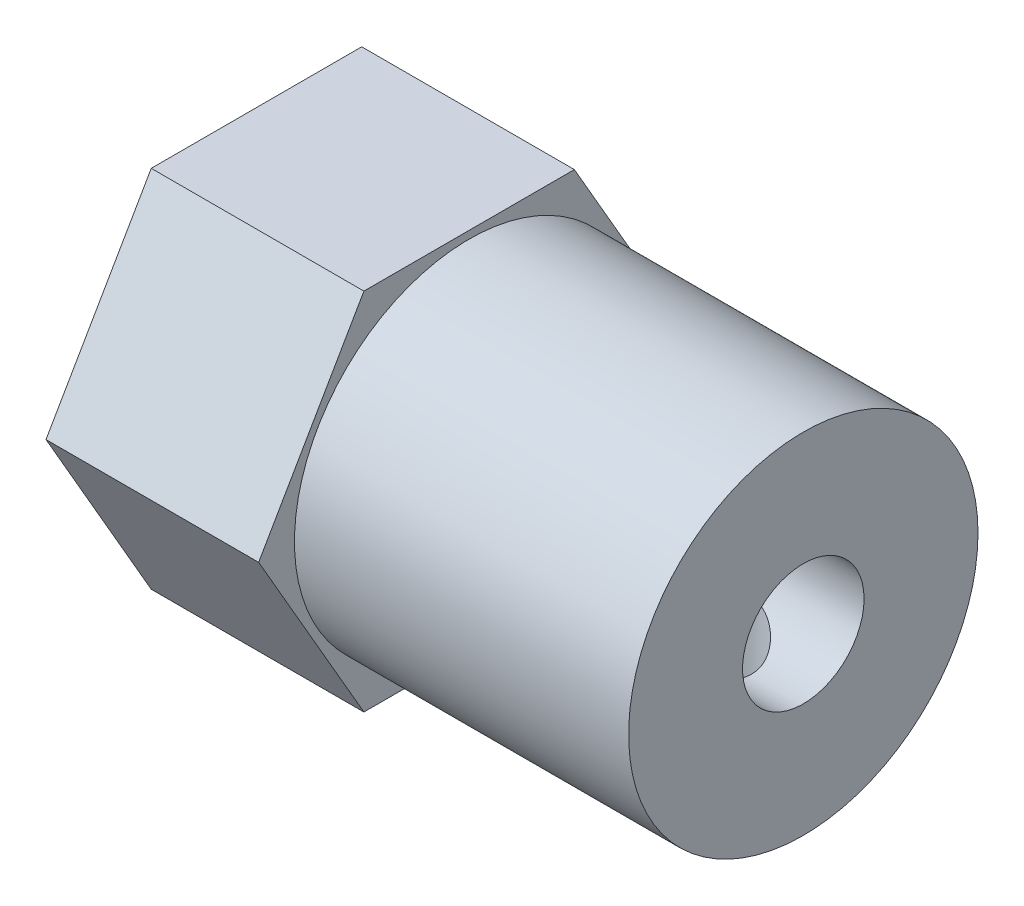
from build123d import *

# Parameters (mm, degrees)
BOSS_EXTRUDE1_DEPTH         = 7
SKETCH2_R                   = 5.75
BOSS_EXTRUDE2_DEPTH         = 11
SKETCH3_R                   = 2
CUT_EXTRUDE1_DEPTH          = 10
M4_TAPPED_HOLE1_D           = 3.3
M4_TAPPED_HOLE1_CSINK_D     = 4.05
M4_TAPPED_HOLE1_CSINK_ANGLE = 90
SKETCH6_R                   = 1.5
CUT_EXTRUDE2_DEPTH          = 21.199009877


with BuildPart() as part:
    # Sketch1 → Boss-Extrude1 (new body)
    with BuildSketch(Plane(origin=(0, 0, 0), x_dir=(0, 0, -1), z_dir=(1, 0, 0))):
        Polygon((6.92820323, 0), (3.464101615, 6), (-3.464101615, 6), (-6.92820323, 0), (-3.464101615, -6), (3.464101615, -6), align=None)
    extrude(amount=BOSS_EXTRUDE1_DEPTH)

    # Sketch2 → Boss-Extrude2 (add)
    with BuildSketch(Plane(origin=(7, 0, 0), x_dir=(0, 0, -1), z_dir=(1, 0, 0))):
        Circle(SKETCH2_R)
    extrude(amount=BOSS_EXTRUDE2_DEPTH)

    # Sketch3 → Cut-Extrude1 (cut)
    with BuildSketch(Plane(origin=(18, 0, 0), x_dir=(0, 0, -1), z_dir=(1, 0, 0))):
        Circle(SKETCH3_R)
    extrude(amount=-CUT_EXTRUDE1_DEPTH, mode=Mode.SUBTRACT)

    # M4 Tapped Hole1 (through all)
    with Locations(Plane.ZY):
        with Locations((0, 0)):
            CounterSinkHole(M4_TAPPED_HOLE1_D / 2, M4_TAPPED_HOLE1_CSINK_D / 2, counter_sink_angle=M4_TAPPED_HOLE1_CSINK_ANGLE)

    # Sketch6 → Cut-Extrude2 (cut, through all)
    with BuildSketch(Plane(origin=(0, 0, 0), x_dir=(1, 0, 0), z_dir=(0, 1, 0))):
        with Locations(Location((14.8, 0, 0), (0, 0, 270))):
            Circle(SKETCH6_R)
    extrude(amount=-CUT_EXTRUDE2_DEPTH, mode=Mode.SUBTRACT)


solid = part.part
